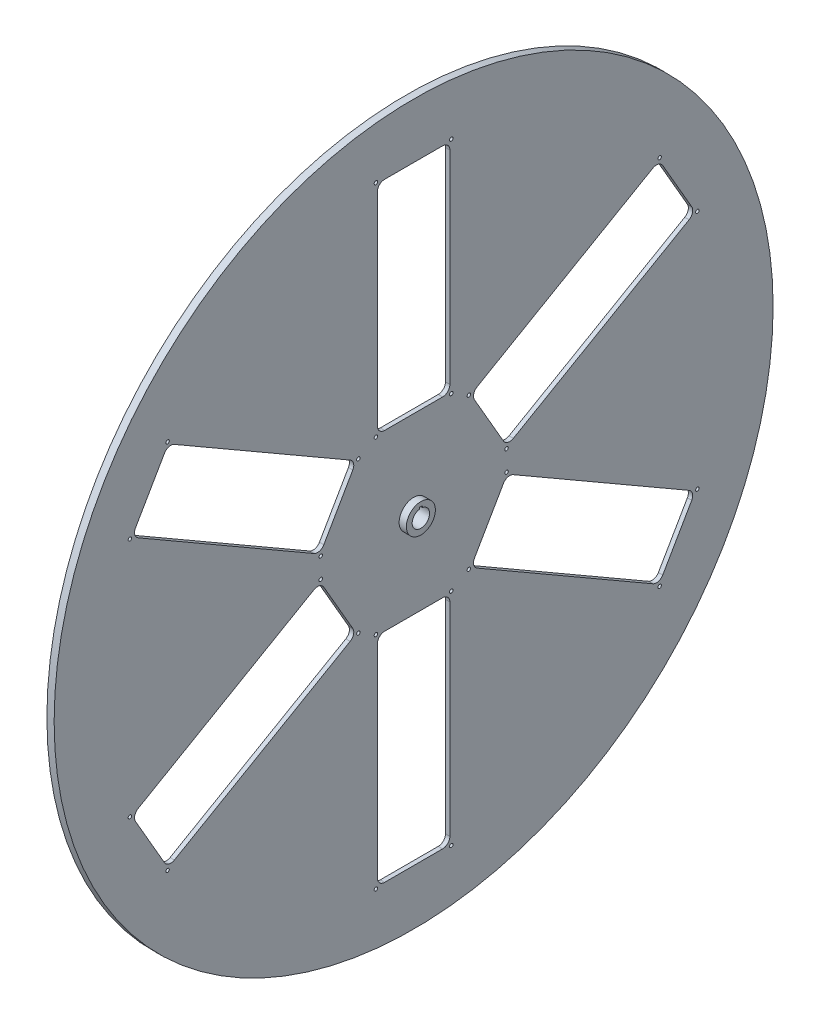
from build123d import *

# Parameters (mm, degrees)
SKETCH1_R                     = 250
BOSS_EXTRUDE1_DEPTH           = 5
SKETCH5_W                     = 50
SKETCH5_H                     = 150
CUT_EXTRUDE1_DEPTH            = 354.588744165
CIRPATTERN1_COUNT             = 6
SKETCH6_W                     = 60
SKETCH6_H                     = 160
CUT_EXTRUDE2_DEPTH            = 2
SKETCH7_R                     = 1
CUT_EXTRUDE3_DEPTH            = 10
M2_CLEARANCE_HOLE1_AT_2_COUNT = 2
M2_CLEARANCE_HOLE1_AT_2_PITCH = 152
M2_CLEARANCE_HOLE1_AT_3_COUNT = 2
M2_CLEARANCE_HOLE1_AT_3_PITCH = 160.648685024
M2_CLEARANCE_HOLE1_AT_4_COUNT = 2
M2_CLEARANCE_HOLE1_AT_4_PITCH = 52
CIRPATTERN2_COUNT             = 6
FILLET1_R                     = 5
FILLET2_R                     = 5
SKETCH11_R                    = 6
CUT_EXTRUDE4_DEPTH            = 354.588744165
BOSS_EXTRUDE2_START           = 5
SKETCH12_R                    = 10
SKETCH12_R_2                  = 6
BOSS_EXTRUDE2_DEPTH           = 15
SKETCH13_W                    = 2
SKETCH13_H                    = 2
CUT_EXTRUDE5_DEPTH            = 354.871445584
SKETCH14_R                    = 250
SKETCH14_R_2                  = 248
CUT_EXTRUDE6_DEPTH            = 354.694783677


with BuildPart() as part:
    # Sketch1 → Boss-Extrude1 (new body)
    with BuildSketch(Plane(origin=(0, 0, 0), x_dir=(0, 0, -1), z_dir=(1, 0, 0))):
        Circle(SKETCH1_R)
    extrude(amount=BOSS_EXTRUDE1_DEPTH)

    # Sketch5 → Cut-Extrude1 (cut, through all)
    with BuildSketch(Plane.ZY):
        with Locations((0, 135)):
            Rectangle(SKETCH5_W, SKETCH5_H)
    cut_extrude1 = extrude(amount=-CUT_EXTRUDE1_DEPTH, mode=Mode.SUBTRACT)

    # CirPattern1: Cut-Extrude1 ×6 about axis
    cirpattern1_axis = Axis((0, 0, 0), (1, 0, 0))
    for i in range(1, CIRPATTERN1_COUNT):
        add(cut_extrude1.rotate(cirpattern1_axis, i * 360 / CIRPATTERN1_COUNT), mode=Mode.SUBTRACT)

    # Sketch6 → Cut-Extrude2 (cut)
    with BuildSketch(Plane.ZY):
        with Locations((0, 135)):
            Rectangle(SKETCH6_W, SKETCH6_H)
    cut_extrude2 = extrude(amount=-CUT_EXTRUDE2_DEPTH, mode=Mode.SUBTRACT)

    # Sketch7 → Cut-Extrude3 (cut)
    with BuildSketch(Plane.ZY.offset(-2)):
        with Locations((-26, 211)):
            Circle(SKETCH7_R)
        with Locations((26, 211)):
            Circle(SKETCH7_R)
        with Locations((-26, 59)):
            Circle(SKETCH7_R)
        with Locations((26, 59)):
            Circle(SKETCH7_R)
    cut_extrude3 = extrude(amount=-CUT_EXTRUDE3_DEPTH, mode=Mode.SUBTRACT)

    # Sketch9 → M2 Clearance Hole1 (revolve, cut)
    with BuildSketch(Plane(origin=(2, 59, -26), x_dir=(0, 0, 1), z_dir=(0, 1, 0))):
        Polygon((0, 0), (0, 8.221032743), (1.2, 7.5), (1.2, 0), align=None)
    m2_clearance_hole1 = revolve(axis=Axis((-4.35, 59, -26), (1, 0, 0)), mode=Mode.SUBTRACT)

    # M2 Clearance Hole1 at 2: M2 Clearance Hole1 ×2
    with Locations(*[(0, i * M2_CLEARANCE_HOLE1_AT_2_PITCH, 0) for i in range(1, M2_CLEARANCE_HOLE1_AT_2_COUNT)]):
        add(m2_clearance_hole1, mode=Mode.SUBTRACT)

    # M2 Clearance Hole1 at 3: M2 Clearance Hole1 ×2
    with Locations(*[Vector(0, 0.9461639849533562, 0.32368767906298995) * (i * M2_CLEARANCE_HOLE1_AT_3_PITCH) for i in range(1, M2_CLEARANCE_HOLE1_AT_3_COUNT)]):
        add(m2_clearance_hole1, mode=Mode.SUBTRACT)

    # M2 Clearance Hole1 at 4: M2 Clearance Hole1 ×2
    with Locations(*[(0, 0, i * M2_CLEARANCE_HOLE1_AT_4_PITCH) for i in range(1, M2_CLEARANCE_HOLE1_AT_4_COUNT)]):
        add(m2_clearance_hole1, mode=Mode.SUBTRACT)

    # CirPattern2: Cut-Extrude2, Cut-Extrude3, M2 Clearance Hole1 ×6 about axis
    cirpattern2_axis = Axis((0, 0, 0), (1, 0, 0))
    add([cut_extrude2.rotate(cirpattern2_axis, i * 360 / CIRPATTERN2_COUNT) for i in range(1, CIRPATTERN2_COUNT)], mode=Mode.SUBTRACT)
    add([cut_extrude3.rotate(cirpattern2_axis, i * 360 / CIRPATTERN2_COUNT) for i in range(1, CIRPATTERN2_COUNT)], mode=Mode.SUBTRACT)
    add([m2_clearance_hole1.rotate(cirpattern2_axis, i * 360 / CIRPATTERN2_COUNT) for i in range(1, CIRPATTERN2_COUNT)], mode=Mode.SUBTRACT)

    # CirPattern2 copy 1 sketch → CirPattern2 copy 1 (revolve, cut)
    with BuildSketch(Plane(origin=(2, 128.016660498, 169.731360199), x_dir=(0, -0.8660254037844386, 0.5000000000000001), z_dir=(0, 0.5000000000000001, 0.8660254037844386))):
        Polygon((0, 0), (0, 8.221032743), (1.2, 7.5), (1.2, 0), align=None)
    revolve(axis=Axis((-4.35, 128.016660498, 169.731360199), (1, 0, 0)), mode=Mode.SUBTRACT)

    # CirPattern2 copy 2 sketch → CirPattern2 copy 2 (revolve, cut)
    with BuildSketch(Plane(origin=(2, -82.983339502, 195.731360199), x_dir=(0, -0.8660254037844387, -0.4999999999999998), z_dir=(0, -0.4999999999999998, 0.8660254037844387))):
        Polygon((0, 0), (0, 8.221032743), (1.2, 7.5), (1.2, 0), align=None)
    revolve(axis=Axis((-4.35, -82.983339502, 195.731360199), (1, 0, 0)), mode=Mode.SUBTRACT)

    # CirPattern2 copy 3 sketch → CirPattern2 copy 3 (revolve, cut)
    with BuildSketch(Plane(origin=(2, -211, 26), x_dir=(0, 0, -1), z_dir=(0, -1, 0))):
        Polygon((0, 0), (0, 8.221032743), (1.2, 7.5), (1.2, 0), align=None)
    revolve(axis=Axis((-4.35, -211, 26), (1, 0, 0)), mode=Mode.SUBTRACT)

    # CirPattern2 copy 4 sketch → CirPattern2 copy 4 (revolve, cut)
    with BuildSketch(Plane(origin=(2, -128.016660498, -169.731360199), x_dir=(0, 0.8660254037844384, -0.5000000000000004), z_dir=(0, -0.5000000000000004, -0.8660254037844384))):
        Polygon((0, 0), (0, 8.221032743), (1.2, 7.5), (1.2, 0), align=None)
    revolve(axis=Axis((-4.35, -128.016660498, -169.731360199), (1, 0, 0)), mode=Mode.SUBTRACT)

    # CirPattern2 copy 5 sketch → CirPattern2 copy 5 (revolve, cut)
    with BuildSketch(Plane(origin=(2, 82.983339502, -195.731360199), x_dir=(0, 0.8660254037844386, 0.5000000000000001), z_dir=(0, 0.5000000000000001, -0.8660254037844386))):
        Polygon((0, 0), (0, 8.221032743), (1.2, 7.5), (1.2, 0), align=None)
    revolve(axis=Axis((-4.35, 82.983339502, -195.731360199), (1, 0, 0)), mode=Mode.SUBTRACT)

    # CirPattern2 copy 6 sketch → CirPattern2 copy 6 (revolve, cut)
    with BuildSketch(Plane(origin=(2, 82.983339502, 195.731360199), x_dir=(0, -0.8660254037844386, 0.5000000000000001), z_dir=(0, 0.5000000000000001, 0.8660254037844386))):
        Polygon((0, 0), (0, 8.221032743), (1.2, 7.5), (1.2, 0), align=None)
    revolve(axis=Axis((-4.35, 82.983339502, 195.731360199), (1, 0, 0)), mode=Mode.SUBTRACT)

    # CirPattern2 copy 7 sketch → CirPattern2 copy 7 (revolve, cut)
    with BuildSketch(Plane(origin=(2, -128.016660498, 169.731360199), x_dir=(0, -0.8660254037844387, -0.4999999999999998), z_dir=(0, -0.4999999999999998, 0.8660254037844387))):
        Polygon((0, 0), (0, 8.221032743), (1.2, 7.5), (1.2, 0), align=None)
    revolve(axis=Axis((-4.35, -128.016660498, 169.731360199), (1, 0, 0)), mode=Mode.SUBTRACT)

    # CirPattern2 copy 8 sketch → CirPattern2 copy 8 (revolve, cut)
    with BuildSketch(Plane(origin=(2, -211, -26), x_dir=(0, 0, -1), z_dir=(0, -1, 0))):
        Polygon((0, 0), (0, 8.221032743), (1.2, 7.5), (1.2, 0), align=None)
    revolve(axis=Axis((-4.35, -211, -26), (1, 0, 0)), mode=Mode.SUBTRACT)

    # CirPattern2 copy 9 sketch → CirPattern2 copy 9 (revolve, cut)
    with BuildSketch(Plane(origin=(2, -82.983339502, -195.731360199), x_dir=(0, 0.8660254037844384, -0.5000000000000004), z_dir=(0, -0.5000000000000004, -0.8660254037844384))):
        Polygon((0, 0), (0, 8.221032743), (1.2, 7.5), (1.2, 0), align=None)
    revolve(axis=Axis((-4.35, -82.983339502, -195.731360199), (1, 0, 0)), mode=Mode.SUBTRACT)

    # CirPattern2 copy 10 sketch → CirPattern2 copy 10 (revolve, cut)
    with BuildSketch(Plane(origin=(2, 128.016660498, -169.731360199), x_dir=(0, 0.8660254037844386, 0.5000000000000001), z_dir=(0, 0.5000000000000001, -0.8660254037844386))):
        Polygon((0, 0), (0, 8.221032743), (1.2, 7.5), (1.2, 0), align=None)
    revolve(axis=Axis((-4.35, 128.016660498, -169.731360199), (1, 0, 0)), mode=Mode.SUBTRACT)

    # CirPattern2 copy 11 sketch → CirPattern2 copy 11 (revolve, cut)
    with BuildSketch(Plane(origin=(2, 6.983339502, 64.095498823), x_dir=(0, -0.8660254037844386, 0.5000000000000001), z_dir=(0, 0.5000000000000001, 0.8660254037844386))):
        Polygon((0, 0), (0, 8.221032743), (1.2, 7.5), (1.2, 0), align=None)
    revolve(axis=Axis((-4.35, 6.983339502, 64.095498823), (1, 0, 0)), mode=Mode.SUBTRACT)

    # CirPattern2 copy 12 sketch → CirPattern2 copy 12 (revolve, cut)
    with BuildSketch(Plane(origin=(2, -52.016660498, 38.095498823), x_dir=(0, -0.8660254037844387, -0.4999999999999998), z_dir=(0, -0.4999999999999998, 0.8660254037844387))):
        Polygon((0, 0), (0, 8.221032743), (1.2, 7.5), (1.2, 0), align=None)
    revolve(axis=Axis((-4.35, -52.016660498, 38.095498823), (1, 0, 0)), mode=Mode.SUBTRACT)

    # CirPattern2 copy 13 sketch → CirPattern2 copy 13 (revolve, cut)
    with BuildSketch(Plane(origin=(2, -59, -26), x_dir=(0, 0, -1), z_dir=(0, -1, 0))):
        Polygon((0, 0), (0, 8.221032743), (1.2, 7.5), (1.2, 0), align=None)
    revolve(axis=Axis((-4.35, -59, -26), (1, 0, 0)), mode=Mode.SUBTRACT)

    # CirPattern2 copy 14 sketch → CirPattern2 copy 14 (revolve, cut)
    with BuildSketch(Plane(origin=(2, -6.983339502, -64.095498823), x_dir=(0, 0.8660254037844384, -0.5000000000000004), z_dir=(0, -0.5000000000000004, -0.8660254037844384))):
        Polygon((0, 0), (0, 8.221032743), (1.2, 7.5), (1.2, 0), align=None)
    revolve(axis=Axis((-4.35, -6.983339502, -64.095498823), (1, 0, 0)), mode=Mode.SUBTRACT)

    # CirPattern2 copy 15 sketch → CirPattern2 copy 15 (revolve, cut)
    with BuildSketch(Plane(origin=(2, 52.016660498, -38.095498823), x_dir=(0, 0.8660254037844386, 0.5000000000000001), z_dir=(0, 0.5000000000000001, -0.8660254037844386))):
        Polygon((0, 0), (0, 8.221032743), (1.2, 7.5), (1.2, 0), align=None)
    revolve(axis=Axis((-4.35, 52.016660498, -38.095498823), (1, 0, 0)), mode=Mode.SUBTRACT)

    # Fillet1
    fillet1_edges = [part.edges().sort_by_distance(p)[0] for p in [
        (1, 55, 30),
        (1, 1.519237886, -62.631397208),
        (1, 81.519237886, -201.195461814),
        (1, 133.480762114, -171.195461814),
        (1, 53.480762114, -32.631397208),
        (1, -53.480762114, -32.631397208),
        (1, -133.480762114, -171.195461814),
        (1, -81.519237886, -201.195461814),
        (1, -1.519237886, -62.631397208),
        (1, -55, 30),
        (1, -215, 30),
        (1, -215, -30),
        (1, -55, -30),
        (1, -1.519237886, 62.631397208),
        (1, -81.519237886, 201.195461814),
        (1, -133.480762114, 171.195461814),
        (1, -53.480762114, 32.631397208),
        (1, 53.480762114, 32.631397208),
        (1, 133.480762114, 171.195461814),
        (1, 81.519237886, 201.195461814),
        (1, 1.519237886, 62.631397208),
        (1, 55, -30),
        (1, 215, -30),
        (1, 215, 30),
    ]]
    fillet(fillet1_edges, radius=FILLET1_R)

    # Fillet2
    fillet2_edges = [part.edges().sort_by_distance(p)[0] for p in [
        (3.5, 60, 25),
        (3.5, 60, -25),
        (3.5, 210, -25),
        (3.5, 126.650635095, -169.365334795),
        (3.5, 51.650635095, -39.461524227),
        (3.5, 8.349364905, -64.461524227),
        (3.5, 83.349364905, -194.365334795),
        (3.5, -83.349364905, -194.365334795),
        (3.5, -8.349364905, -64.461524227),
        (3.5, -51.650635095, -39.461524227),
        (3.5, -126.650635095, -169.365334795),
        (3.5, -210, -25),
        (3.5, -60, -25),
        (3.5, -60, 25),
        (3.5, -210, 25),
        (3.5, -126.650635095, 169.365334795),
        (3.5, -51.650635095, 39.461524227),
        (3.5, -8.349364905, 64.461524227),
        (3.5, -83.349364905, 194.365334795),
        (3.5, 83.349364905, 194.365334795),
        (3.5, 8.349364905, 64.461524227),
        (3.5, 51.650635095, 39.461524227),
        (3.5, 126.650635095, 169.365334795),
        (3.5, 210, 25),
    ]]
    fillet(fillet2_edges, radius=FILLET2_R)

    # Sketch11 → Cut-Extrude4 (cut, through all)
    with BuildSketch(Plane.ZY):
        Circle(SKETCH11_R)
    extrude(amount=-CUT_EXTRUDE4_DEPTH, mode=Mode.SUBTRACT)

    # Sketch12 → Boss-Extrude2 (add)
    with BuildSketch(Plane.ZY.offset(BOSS_EXTRUDE2_START)):
        Circle(SKETCH12_R)
        Circle(SKETCH12_R_2, mode=Mode.SUBTRACT)
    extrude(amount=-BOSS_EXTRUDE2_DEPTH)

    # Sketch13 → Cut-Extrude5 (cut, through all)
    with BuildSketch(Plane.ZY.offset(5)):
        with Locations((0, 6)):
            Rectangle(SKETCH13_W, SKETCH13_H)
    extrude(amount=-CUT_EXTRUDE5_DEPTH, mode=Mode.SUBTRACT)

    # Sketch14 → Cut-Extrude6 (cut, through all)
    with BuildSketch(Plane.ZY):
        Circle(SKETCH14_R)
        Circle(SKETCH14_R_2, mode=Mode.SUBTRACT)
    extrude(amount=-CUT_EXTRUDE6_DEPTH, mode=Mode.SUBTRACT)


solid = part.part
